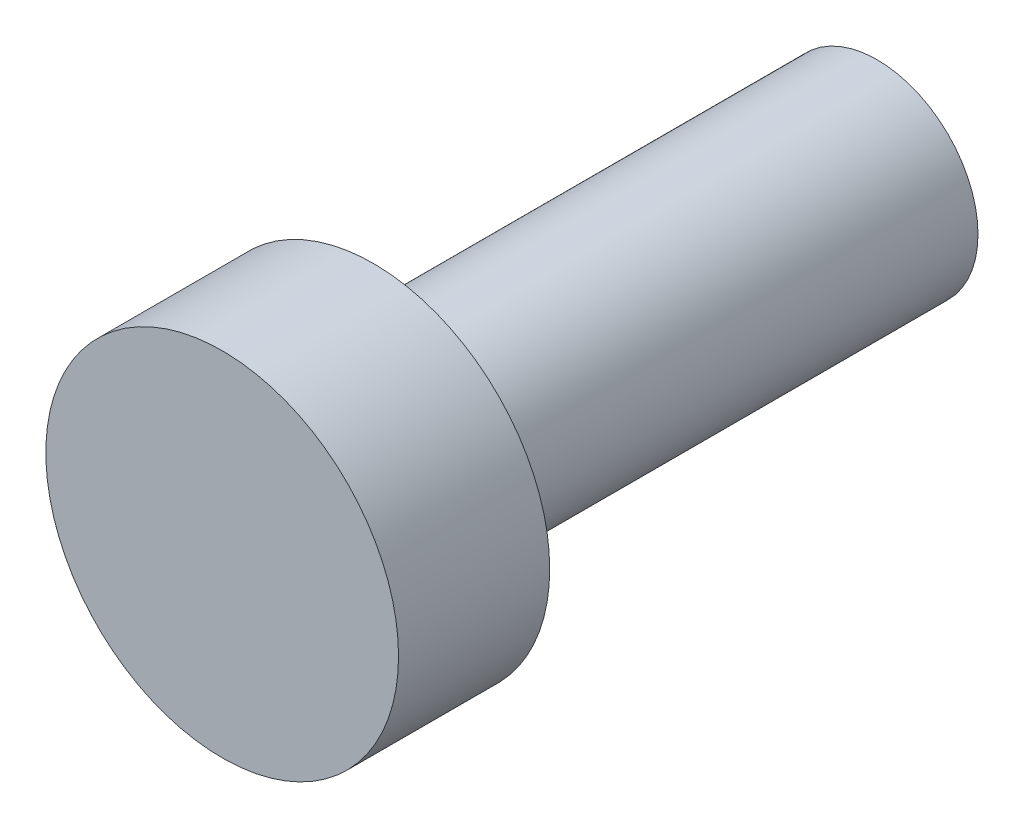
from build123d import *

# Parameters (mm, degrees)
SKETCH_1_R      = 2
EXTRUDE_1_DEPTH = 10
SKETCH_2_R      = 3.5
EXTRUDE_2_DEPTH = 3


with BuildPart() as part:
    # 草图1 → 凸台-拉伸1 (new body)
    with BuildSketch(Plane.XY):
        Circle(SKETCH_1_R)
    extrude(amount=-EXTRUDE_1_DEPTH)

    # 草图2 → 凸台-拉伸2 (add)
    with BuildSketch(Plane.XY):
        Circle(SKETCH_2_R)
    extrude(amount=EXTRUDE_2_DEPTH)


solid = part.part
